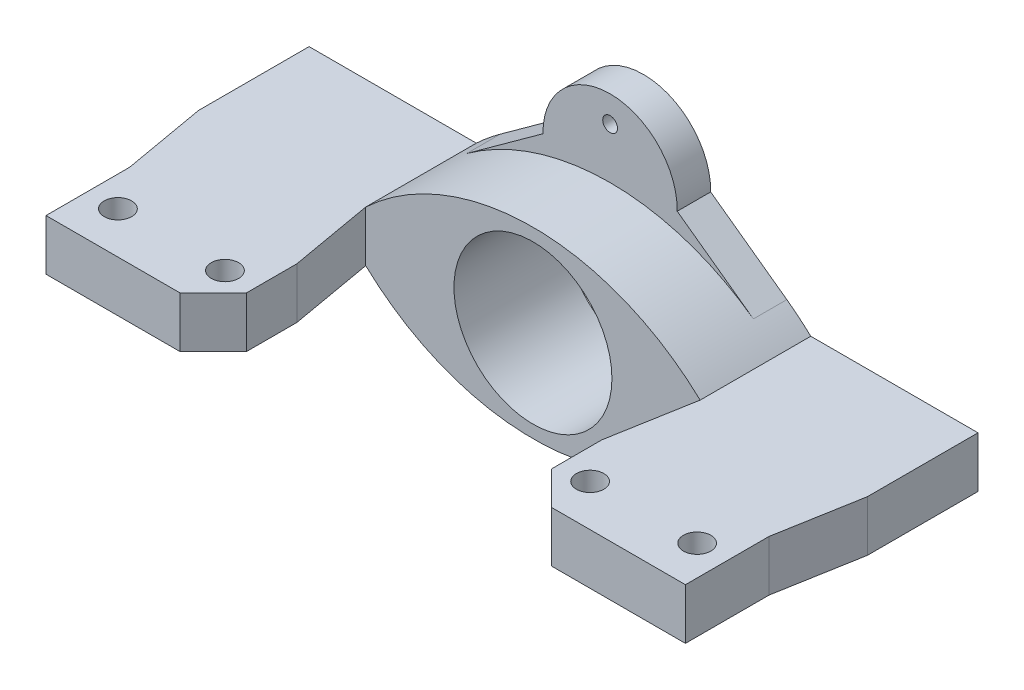
from build123d import *

# Parameters (mm, degrees)
SKETCH1_W           = 127
SKETCH1_H           = 38.1
SKETCH1_R           = 15
BOSS_EXTRUDE1_DEPTH = 21
BOSS_EXTRUDE2_DEPTH = 6.35
SKETCH4_R           = 1.4
CUT_EXTRUDE2_DEPTH  = 6.35
CUT_EXTRUDE6_DEPTH  = 14.65
CUT_EXTRUDE7_DEPTH  = 73.600774789
SKETCH7_R           = 2.6035
CUT_EXTRUDE8_DEPTH  = 22.86
SKETCH8_W           = 31.75
SKETCH8_H           = 15.875
SKETCH8_R           = 2.6035
BOSS_EXTRUDE3_DEPTH = 9.652
CHAMFER1_SIZE       = 6.35
BOSS_EXTRUDE4_START = -9.652
SKETCH9_W           = 26.681402361
SKETCH9_H           = 11.886393241
SKETCH9_R           = 2.6035
SKETCH9_W_2         = 26.993648234
BOSS_EXTRUDE4_DEPTH = 9.652


with BuildPart() as part:
    # Sketch1 → Boss-Extrude1 (new body)
    with BuildSketch(Plane.XY):
        Rectangle(SKETCH1_W, SKETCH1_H)
        Circle(SKETCH1_R, mode=Mode.SUBTRACT)
    extrude(amount=-BOSS_EXTRUDE1_DEPTH)

    # Sketch3 → Boss-Extrude2 (add)
    with BuildSketch(Plane(origin=(0, 0, -21), x_dir=(-1, 0, 0), z_dir=(0, 0, -1))):
        with BuildLine():
            Line((12.743745366, -19.05), (-12.743745366, -19.05))
            ThreePointArc((-12.743745366, -19.05), (-9.084403439, -28.194328353), (1.02e-07, -32))
            ThreePointArc((1.02e-07, -32), (9.08440351, -28.194328281), (12.743745366, -19.05))
        make_face()
    boss_extrude2 = extrude(amount=-BOSS_EXTRUDE2_DEPTH)

    # Sketch4 → Cut-Extrude2 (cut)
    with BuildSketch(Plane.XY.offset(-14.65)):
        with Locations((0, -27)):
            Circle(SKETCH4_R)
    cut_extrude2 = extrude(amount=-CUT_EXTRUDE2_DEPTH, mode=Mode.SUBTRACT)

    # Mirror1: Boss-Extrude2, Cut-Extrude2 across plane
    add(boss_extrude2.mirror(Plane.ZX))
    add(cut_extrude2.mirror(Plane.ZX), mode=Mode.SUBTRACT)

    # Sketch5 → Cut-Extrude6 (cut)
    with BuildSketch(Plane.XY):
        with BuildLine():
            Line((-31.75, -4.826), (-63.5, -4.826))
            Line((-63.5, -4.826), (-63.5, -19.05))
            Line((-63.5, -19.05), (63.5, -19.05))
            Line((63.5, -19.05), (63.5, -4.826))
            Line((63.5, -4.826), (31.75, -4.826))
            ThreePointArc((31.75, -4.826), (0, -17.39350594), (-31.75, -4.826))
        make_face()
        with BuildLine():
            Line((-63.5, 19.05), (-63.5, 4.826))
            Line((-63.5, 4.826), (-31.75, 4.826))
            ThreePointArc((-31.75, 4.826), (0, 17.39350594), (31.75, 4.826))
            Line((31.75, 4.826), (63.5, 4.826))
            Line((63.5, 4.826), (63.5, 19.05))
            Line((63.5, 19.05), (-63.5, 19.05))
        make_face()
    extrude(amount=-CUT_EXTRUDE6_DEPTH, mode=Mode.SUBTRACT)

    # Sketch6 → Cut-Extrude7 (cut, through all)
    with BuildSketch(Plane.XY.offset(-14.65)):
        with BuildLine():
            Line((27.206467014, -8.577889412), (12.743745366, -19.05))
            Line((12.743745366, -19.05), (63.5, -19.05))
            Line((63.5, -19.05), (63.5, -4.826))
            Line((63.5, -4.826), (31.75, -4.826))
            ThreePointArc((31.75, -4.826), (29.537864162, -6.774157348), (27.206467014, -8.577889412))
        make_face()
        with BuildLine():
            Line((-63.5, -19.05), (-12.743745366, -19.05))
            Line((-12.743745366, -19.05), (-27.206467014, -8.577889412))
            ThreePointArc((-27.206467014, -8.577889412), (-29.537864162, -6.774157348), (-31.75, -4.826))
            Line((-31.75, -4.826), (-63.5, -4.826))
            Line((-63.5, -4.826), (-63.5, -19.05))
        make_face()
        with BuildLine():
            Line((-27.206467014, 8.577889412), (-12.743745366, 19.05))
            Line((-12.743745366, 19.05), (-63.5, 19.05))
            Line((-63.5, 19.05), (-63.5, 4.826))
            Line((-63.5, 4.826), (-31.75, 4.826))
            ThreePointArc((-31.75, 4.826), (-29.537864162, 6.774157348), (-27.206467014, 8.577889412))
        make_face()
        with BuildLine():
            Line((63.5, 19.05), (12.743745366, 19.05))
            Line((12.743745366, 19.05), (27.206467014, 8.577889412))
            ThreePointArc((27.206467014, 8.577889412), (29.537864162, 6.774157348), (31.75, 4.826))
            Line((31.75, 4.826), (63.5, 4.826))
            Line((63.5, 4.826), (63.5, 19.05))
        make_face()
    extrude(amount=-CUT_EXTRUDE7_DEPTH, mode=Mode.SUBTRACT)

    # Sketch7 → Cut-Extrude8 (cut)
    with BuildSketch(Plane(origin=(0, 4.826, 0), x_dir=(1, 0, 0), z_dir=(0, 1, 0))):
        with Locations(Location((-57.785, 10.5, 0), (0, 0, 270))):
            Circle(SKETCH7_R)
        with Locations(Location((-37.465, 10.5, 0), (0, 0, 270))):
            Circle(SKETCH7_R)
        with Locations(Location((37.465, 10.5, 0), (0, 0, 270))):
            Circle(SKETCH7_R)
        with Locations(Location((57.785, 10.5, 0), (0, 0, 270))):
            Circle(SKETCH7_R)
    extrude(amount=-CUT_EXTRUDE8_DEPTH, mode=Mode.SUBTRACT)

    # Sketch8 → Boss-Extrude3 (add)
    # profile 1 of 4: a face of its own
    with BuildSketch(Plane.XZ.offset(4.826)):
        Polygon((63.5, 0), (31.75, 0), (28.950809181, 15.875), (60.700809181, 15.875), align=None)
    # profile 2 of 4: a face of its own
    with BuildSketch(Plane.XZ.offset(4.826)):
        with Locations((44.825809181, 23.8125)):
            Rectangle(SKETCH8_W, SKETCH8_H)
        with Locations(Location((34.665809181, 23.8125, 0), (0, 0, 270))):
            Circle(SKETCH8_R, mode=Mode.SUBTRACT)
        with Locations(Location((54.985809181, 23.8125, 0), (0, 0, 270))):
            Circle(SKETCH8_R, mode=Mode.SUBTRACT)
    # profile 3 of 4: a face of its own
    with BuildSketch(Plane.XZ.offset(4.826)):
        with Locations((-44.825809181, 23.8125)):
            Rectangle(SKETCH8_W, SKETCH8_H)
        with Locations(Location((-34.665809181, 23.8125, 0), (0, 0, 270))):
            Circle(SKETCH8_R, mode=Mode.SUBTRACT)
        with Locations(Location((-54.985809181, 23.8125, 0), (0, 0, 270))):
            Circle(SKETCH8_R, mode=Mode.SUBTRACT)
    # profile 4 of 4: a face of its own
    with BuildSketch(Plane.XZ.offset(4.826)):
        Polygon((-60.700809181, 15.875), (-28.950809181, 15.875), (-31.75, 0), (-63.5, 0), align=None)
    extrude(amount=-BOSS_EXTRUDE3_DEPTH)

    # Chamfer1
    chamfer1_edges = [part.edges().sort_by_distance(p)[0] for p in [
        (28.950809181, 0, 31.75),
        (-28.950809181, 0, 31.75),
    ]]
    chamfer(chamfer1_edges, length=CHAMFER1_SIZE)

    # Sketch9 → Boss-Extrude4 (add)
    # profile 1 of 4: a face of its own
    with BuildSketch(Plane.XZ.offset(4.826).offset(BOSS_EXTRUDE4_START)):
        with Locations((-47.360108001, -9.539491199)):
            Rectangle(SKETCH9_W, SKETCH9_H)
        with Locations((-57.785, -10.5)):
            Circle(SKETCH9_R, mode=Mode.SUBTRACT)
        with Locations((-37.465, -10.5)):
            Circle(SKETCH9_R, mode=Mode.SUBTRACT)
    # profile 2 of 4: a face of its own
    with BuildSketch(Plane.XZ.offset(4.826).offset(BOSS_EXTRUDE4_START)):
        with Locations((-57.785, -10.5)):
            Circle(SKETCH9_R)
    # profile 3 of 4: a face of its own
    with BuildSketch(Plane.XZ.offset(4.826).offset(BOSS_EXTRUDE4_START)):
        with Locations((-37.465, -10.5)):
            Circle(SKETCH9_R)
    # profile 4 of 4: a face of its own
    with BuildSketch(Plane.XZ.offset(4.826).offset(BOSS_EXTRUDE4_START)):
        with Locations((47.713125711, -9.539491199)):
            Rectangle(SKETCH9_W_2, SKETCH9_H)
    extrude(amount=BOSS_EXTRUDE4_DEPTH)


solid = part.part
